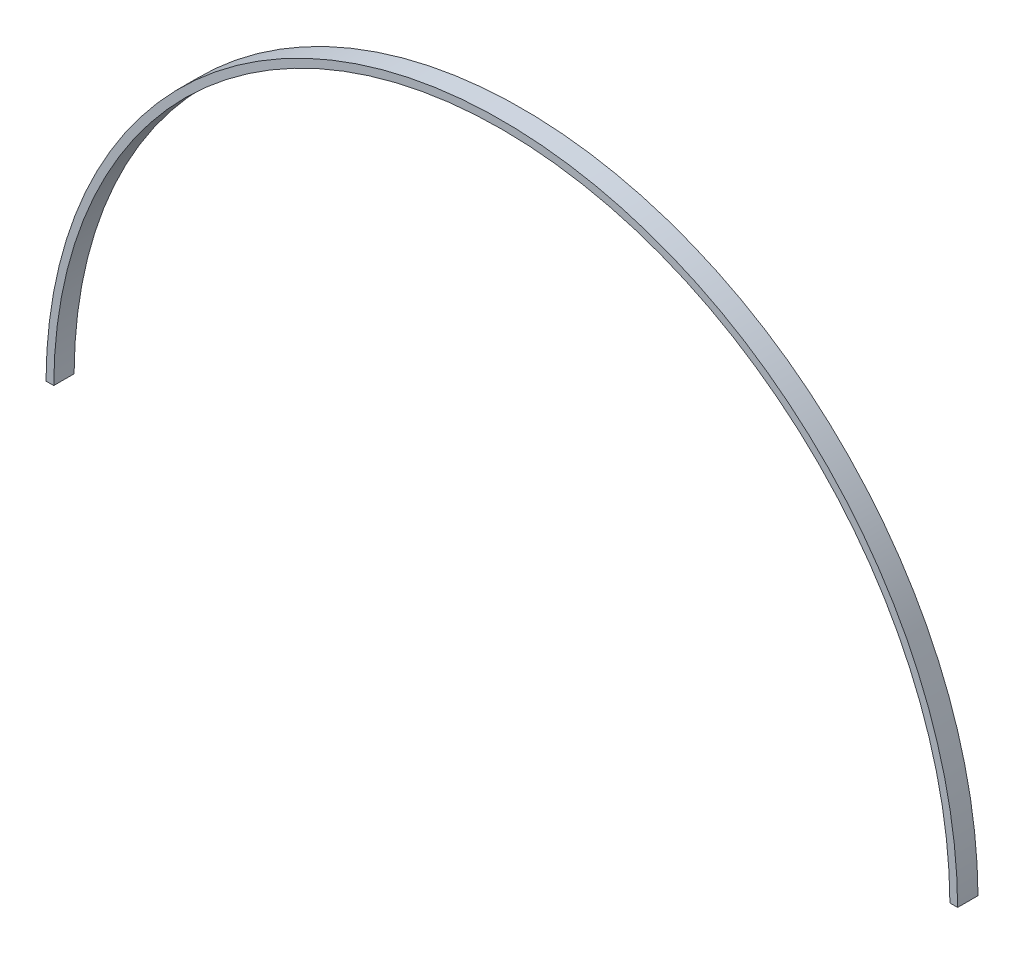
SolidWorks part; units mm, degrees
ref_plane "前视基准面" through (0, 0, 0) normal (0, 0, 1) x (1, 0, 0)
ref_plane "上视基准面" through (0, 0, 0) normal (0, 1, 0) x (1, 0, 0)
ref_plane "右视基准面" through (0, 0, 0) normal (1, 0, 0) x (0, 0, -1)
other "Configuration Table"
sketch "草图1" plane through (0, 0, 0) normal (0, 0, 1) x (1, 0, 0)
  line L0 (-3.9978, 1) -> (-0.1977, 1)
  line L1 (440.1977, 1) -> (443.9978, 1)
  arc A0 (443.9978, 1) -> (-3.9978, 1) centre (220, 0) ccw
  arc A1 (-0.1977, 1) -> (440.1977, 1) centre (220, 0) cw
  point P0 (0, 0)
  dimension "D1" = 224
  dimension "D2" = 220.2
  dimension "D3" = 3.8
  dimension "D4" = 443.9978
extrude "凸台-拉伸1" add sketch "草图1" against normal mid plane 10
